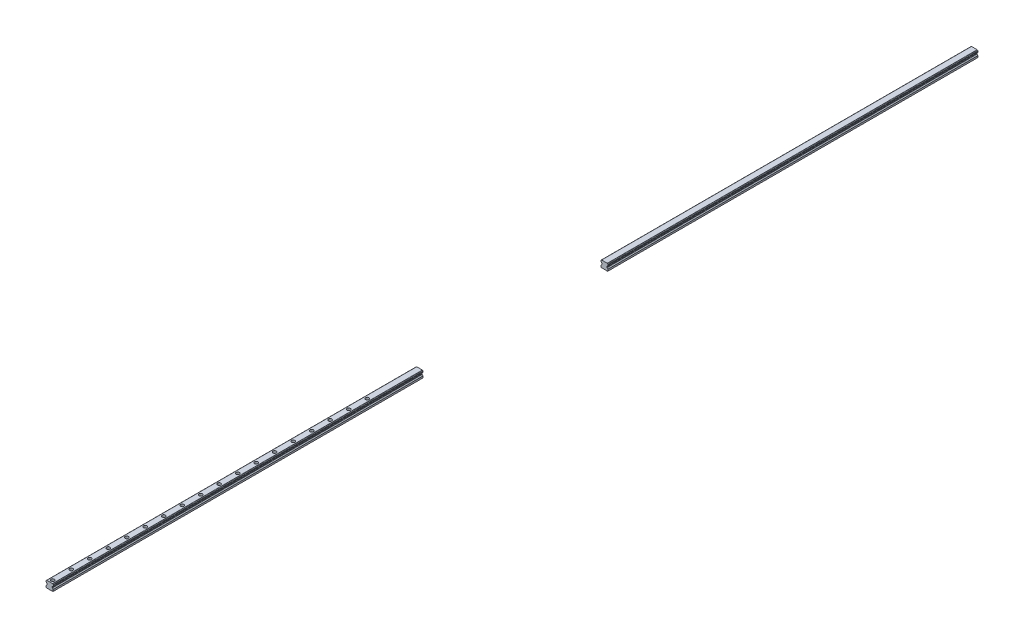
from build123d import *

# Parameters (mm, degrees)
BOSS_EXTRUDE1_DEPTH           = 3000
COUNTERBORE_HOLE1_D           = 7
COUNTERBORE_HOLE1_CBORE_D     = 11
COUNTERBORE_HOLE1_CBORE_DEPTH = 9
LPATTERN1_COUNT               = 18
LPATTERN1_PITCH               = 60
CHAMFER1_SIZE                 = 1
SKETCH7_W                     = 717.319877582
SKETCH7_H                     = 600
CUT_EXTRUDE1_DEPTH            = 3001.104383984


with BuildPart() as part:
    # Sketch3 → Boss-Extrude1 (new body)
    with BuildSketch(Plane.XY):
        with BuildLine():
            Line((-11.5, -6.5), (11.5, -6.5))
            Line((11.5, -6.5), (11.5, 0))
            Line((11.5, 0), (8.738819621, 2.761180379))
            ThreePointArc((8.738819621, 2.761180379), (8.420886253, 3.23700129), (8.309242901, 3.798270324))
            Line((8.309242901, 3.798270324), (8.309242901, 5.792910054))
            ThreePointArc((8.309242901, 5.792910054), (8.420886253, 6.354179088), (8.738819621, 6.83))
            Line((8.738819621, 6.83), (11.5, 9.591180379))
            ThreePointArc((11.5, 9.591180379), (11.817933369, 10.06700129), (11.929576721, 10.628270324))
            Line((11.929576721, 10.628270324), (11.929576721, 12.622910054))
            ThreePointArc((11.929576721, 12.622910054), (11.817933369, 13.184179088), (11.5, 13.66))
            Line((11.5, 13.66), (10.089576721, 15.070423279))
            ThreePointArc((10.089576721, 15.070423279), (9.613755809, 15.388356648), (9.052486775, 15.5))
            Line((9.052486775, 15.5), (-9.052486775, 15.5))
            ThreePointArc((-9.052486775, 15.5), (-9.613755809, 15.388356648), (-10.089576721, 15.070423279))
            Line((-10.089576721, 15.070423279), (-11.5, 13.66))
            ThreePointArc((-11.5, 13.66), (-11.817933369, 13.184179088), (-11.929576721, 12.622910054))
            Line((-11.929576721, 12.622910054), (-11.929576721, 10.628270324))
            ThreePointArc((-11.929576721, 10.628270324), (-11.817933369, 10.06700129), (-11.5, 9.591180379))
            Line((-11.5, 9.591180379), (-8.738819621, 6.83))
            ThreePointArc((-8.738819621, 6.83), (-8.420886253, 6.354179088), (-8.309242901, 5.792910054))
            Line((-8.309242901, 5.792910054), (-8.309242901, 3.798270324))
            ThreePointArc((-8.309242901, 3.798270324), (-8.420886253, 3.23700129), (-8.738819621, 2.761180379))
            Line((-8.738819621, 2.761180379), (-11.5, 0))
            Line((-11.5, 0), (-11.5, -6.5))
        make_face()
    extrude(amount=-BOSS_EXTRUDE1_DEPTH)

    # Counterbore Hole1 (through all)
    with Locations(Plane(origin=(0, 15.5, 0), x_dir=(-1, 0, 0), z_dir=(0, 1, 0))):
        with Locations((0, -10)):
            counterbore_hole1 = CounterBoreHole(COUNTERBORE_HOLE1_D / 2, COUNTERBORE_HOLE1_CBORE_D / 2, COUNTERBORE_HOLE1_CBORE_DEPTH)

    # LPattern1: Counterbore Hole1 ×18
    with Locations(*[(0, 0, -i * LPATTERN1_PITCH) for i in range(1, LPATTERN1_COUNT)]):
        add(counterbore_hole1, mode=Mode.SUBTRACT)

    # Chamfer1
    chamfer1_edges = [part.edges().sort_by_distance(p)[0] for p in [
        (11.5, -6.5, -1500),
        (-11.5, -6.5, -1500),
    ]]
    chamfer(chamfer1_edges, length=CHAMFER1_SIZE)

    # Sketch7 → Cut-Extrude1 (cut, through all)
    with BuildSketch(Plane(origin=(0, 15.5, 0), x_dir=(1, 0, 0), z_dir=(0, 1, 0))):
        with Locations((-6.404641764, 1500)):
            Rectangle(SKETCH7_W, SKETCH7_H)
    extrude(amount=-CUT_EXTRUDE1_DEPTH, mode=Mode.SUBTRACT)


with BuildPart() as cut_extrude1_piece_1:
    # of the separate pieces the step leaves, piece 1, a body of its own (cut_extrude1_pieces)
    add(part.part.solids().sort_by_distance((-11.5, -5.5, -1800))[0])


with BuildPart() as cut_extrude1_piece_2:
    # of the separate pieces the step leaves, piece 2, a body of its own (cut_extrude1_pieces)
    add(part.part.solids().sort_by_distance((-11.5, -5.5, 0))[0])


solid = Compound([cut_extrude1_piece_1.part, cut_extrude1_piece_2.part])
